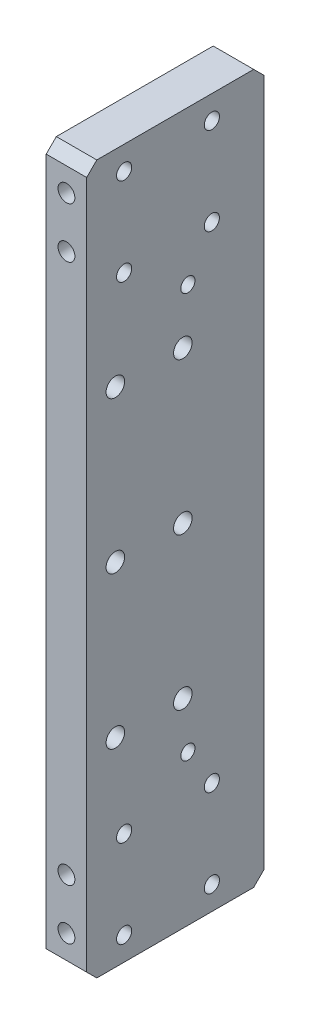
SolidWorks part; units mm, degrees
material "6061 Alloy"
ref_plane "Front Plane" through (0, 0, 0) normal (0, 0, 1) x (1, 0, 0)
ref_plane "Top Plane" through (0, 0, 0) normal (0, 1, 0) x (1, 0, 0)
ref_plane "Right Plane" through (0, 0, 0) normal (1, 0, 0) x (0, 0, -1)
sketch "Sketch 1" plane through (0, 0, 0) normal (1, 0, 0) x (0, 0, -1)
  line L1 (-34, -95) -> (34, -95)
  line L2 (-34, -95) -> (-34, 95)
  line L3 (-34, 95) -> (34, 95)
  line L4 (34, -95) -> (34, 95)
  line L5 (-34, -95) -> (34, 95) construction
  line L6 (-34, 95) -> (34, -95) construction
  point P0 (0, 0)
  dimension "D1" = 68
  dimension "D2" = 190
extrude "Boss-Extrude 1" add sketch "Sketch 1" along normal blind 12
sketch "Sketch 9" plane through (0, 0, 0) normal (-1, 0, 0) x (0, 0, 1)
  line L1 (34, 95) -> (-34, 95)
  line L2 (34, 95) -> (34, 105)
  line L3 (34, 105) -> (-34, 105)
  line L4 (-34, 95) -> (-34, 105)
  line L5 (34, -95) -> (-34, -95)
  line L6 (34, -95) -> (34, -105)
  line L7 (34, -105) -> (-34, -105)
  line L8 (-34, -95) -> (-34, -105)
  dimension "D1" = 68
  dimension "D2" = 68
  dimension "D3" = 10
  dimension "D4" = 10
extrude "Boss-Extrude 2" add sketch "Sketch 9" against normal blind 12
hole_wizard "Ø4.5 (4.5) Hole 1" positions "Sketch 11" profile "Sketch 10" hole size "Ø4.5" standard "JIS" end condition through all
sketch "Sketch 11" plane through (0, 0, 0) normal (-1, 0, 0) x (0, 0, 1)
  line L0 (-34, -105) -> (34, -105) construction
  line L1 (34, 105) -> (34, -105) construction
  point P0 (22.9, -98)
  dimension "D1" = 7
  dimension "D2" = 11.1
sketch "Sketch 10" plane through (0, -98, 22.9) normal (0, 1, 0) x (0, 0, 1)
  line L0 (0, 0) -> (0, 12)
  line L1 (0, 12) -> (2.25, 12)
  line L2 (2.25, 12) -> (2.25, 0)
  line L5 (2.25, 0) -> (0, 0)
  line L11 (0, -6.35) -> (0, 107.95) construction
  dimension "貫穿孔直徑" = 4.5
  dimension "貫穿孔深度" = 12
pattern_linear "Linear Pattern 2" count 2 spacing 26 along (0, 1, 0) count 2 spacing 26 along (0, 0, -1) of "Ø4.5 (4.5) Hole 1"
hole_wizard "M5 Socket Head Cap Screw Counterbore 1" positions "Sketch 13" profile "Sketch 12" counterbore size "M5" standard "JIS" end condition through all
sketch "Sketch 13" plane through (0, 0, 0) normal (-1, 0, 0) x (0, 0, 1)
  line L1 (34, 105) -> (-34, 105) construction
  line L2 (-34, -105) -> (-34, 105) construction
  point P0 (5.5, 44)
  dimension "D1" = 39.5
  dimension "D2" = 61
sketch "Sketch 12" plane through (0, 44, 5.5) normal (0, 1, 0) x (0, 0, 1)
  line L0 (0, 0) -> (0, 12)
  line L1 (0, 12) -> (2.75, 12)
  line L3 (2.75, 12) -> (2.75, 5)
  line L4 (2.75, 5) -> (5, 5)
  line L5 (5, 5) -> (5, 0)
  line L7 (5, 0) -> (0, 0)
  line L11 (0, -6.35) -> (0, 107.95) construction
  dimension "貫穿孔直徑" = 5.5
  dimension "貫穿孔深度" = 12
  dimension "柱孔直徑" = 10
  dimension "柱孔深度" = 5
pattern_linear "Linear Pattern 3" count 3 spacing 45 along (0, -1, 0) count 2 spacing 20 along (0, 0, 1) of "M5 Socket Head Cap Screw Counterbore 1"
sketch "Sketch 14" plane through (0, 0, 0) normal (-1, 0, 0) x (0, 0, 1)
  line L0 (34, 105) -> (-34, 105) construction
  line L1 (-18.5, 105) -> (-38.5, 105)
  line L2 (-18.5, 105) -> (-18.5, -110)
  line L3 (-18.5, -110) -> (-38.5, -110)
  line L4 (-38.5, 105) -> (-38.5, -110)
  line L5 (-34, -105) -> (-34, 105) construction
  dimension "D1" = 20
  dimension "D2" = 15.5
  dimension "D3" = 215
extrude "Cut-Extrude 4" cut sketch "Sketch 14" against normal through all
pattern_linear "Linear Pattern 4" count 2 spacing 170 along (0, 1, 0) of "Linear Pattern 2", "Ø4.5 (4.5) Hole 1"
hole_wizard "M5 Tapped Hole 1" positions "Sketch 16" profile "Sketch 15" tap size "M5" standard "GB" end condition through all
sketch "Sketch 16" plane through (0, 0, 0) normal (-1, 0, 0) x (0, 0, 1)
  line L0 (-18.5, -105) -> (-18.5, 105) construction
  line L1 (34, 105) -> (-18.5, 105) construction
  point P0 (4, 59.5)
  dimension "D1" = 22.5
  dimension "D2" = 45.5
sketch "Sketch 15" plane through (0, 59.5, 4) normal (0, 1, 0) x (0, 0, 1)
  line L0 (0, 0) -> (0, 12)
  line L1 (0, 12) -> (2.1, 12)
  line L2 (2.1, 12) -> (2.1, 0)
  line L5 (2.1, 0) -> (0, 0)
  line L11 (0, -6.35) -> (0, 107.95) construction
  dimension "貫穿螺孔鑽直徑" = 4.2
  dimension "貫穿螺孔鑽深度" = 12
cosmetic thread "Cosmetic Thread 1" parameters "D2"=5
pattern_linear "Linear Pattern 5" count 2 spacing 120 along (0, -1, 0) of "M5 Tapped Hole 1"
hole_wizard "M6 Tapped Hole 1" positions "Sketch 18" profile "Sketch 17" tap size "M6" standard "GB"
sketch "Sketch 18" plane through (0, 0, 34) normal (0, 0, 1) x (1, 0, 0)
  line L0 (12, 105) -> (12, -105) construction
  line L1 (12, 105) -> (0, 105) construction
  point P0 (6, 95)
  dimension "D1" = 6
  dimension "D2" = 10
sketch "Sketch 17" plane through (6, 95, 34) normal (1, 0, 0) x (0, -1, 0)
  line L0 (0, 0) -> (0, 16.5022)
  line L1 (0, 16.5022) -> (2.5, 15)
  line L2 (2.5, 15) -> (2.5, 0)
  line L5 (2.5, 0) -> (0, 0)
  line L10 (0, 16.5022) -> (-2.5, 15) construction
  line L11 (0, -6.35) -> (0, 107.95) construction
  dimension "螺孔鑽直徑" = 5
  dimension "螺孔鑽深度" = 15
  dimension "導頭角度" = 118
cosmetic thread "Cosmetic Thread 2" parameters "D1"=12, "D2"=6
pattern_linear "Linear Pattern 6" count 2 spacing 15 along (0, -1, 0) of "M6 Tapped Hole 1"
mirror "Mirror 1" about plane through (0, 0, 0) normal (0, 1, 0) of "Linear Pattern 6", "M6 Tapped Hole 1"
chamfer "Chamfer 1" distance 3 angle 45 4 edges at (6, -105, 34) (6, -105, -18.5) (6, 105, -18.5) (6, 105, 34)
